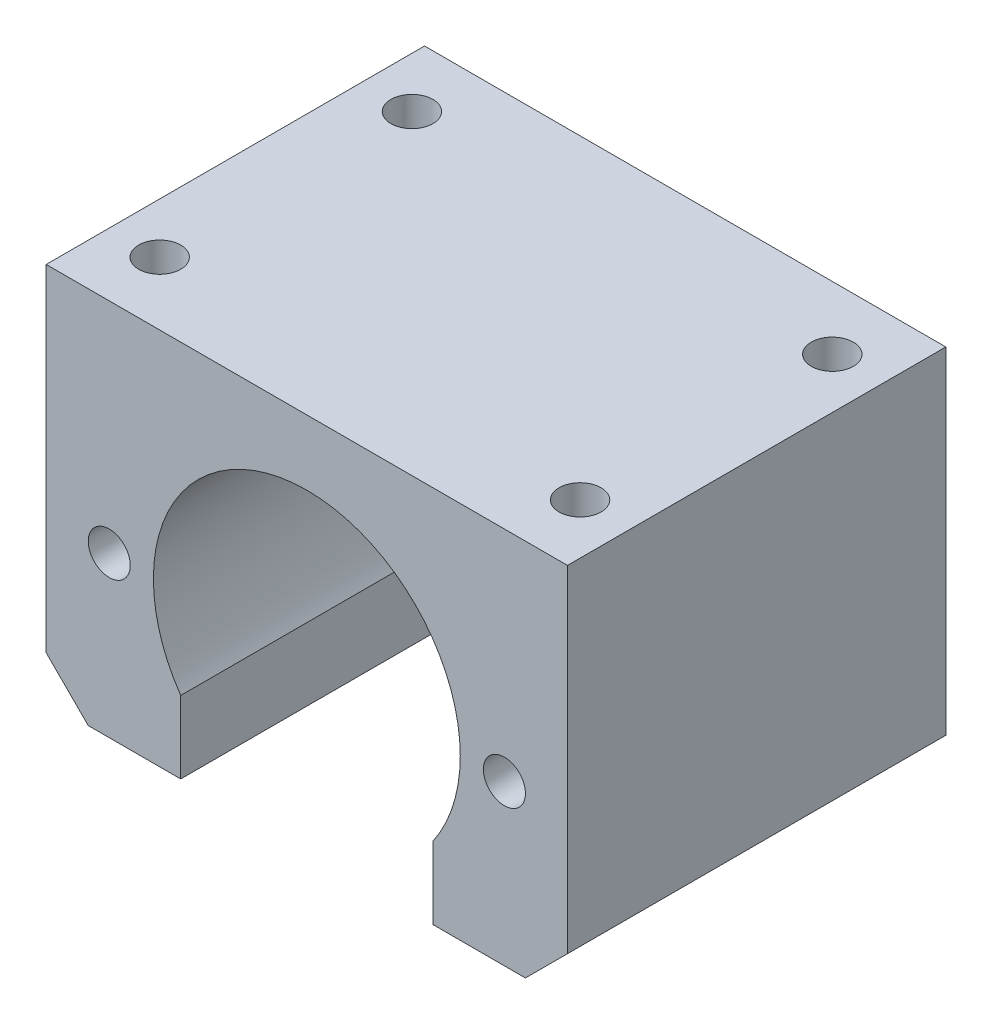
SolidWorks part; units mm, degrees
material "A6061"
ref_plane "前基準面" through (0, 0, 0) normal (0, 0, 1) x (1, 0, 0)
ref_plane "上基準面" through (0, 0, 0) normal (0, 1, 0) x (1, 0, 0)
ref_plane "右基準面" through (0, 0, 0) normal (1, 0, 0) x (0, 0, -1)
sketch "草图1" plane through (0, 0, 0) normal (0, 1, 0) x (1, 0, 0)
  line L1 (-31, -22.5) -> (31, -22.5)
  line L2 (-31, -22.5) -> (-31, 22.5)
  line L3 (-31, 22.5) -> (31, 22.5)
  line L4 (31, -22.5) -> (31, 22.5)
  line L5 (-31, -22.5) -> (31, 22.5) construction
  line L6 (-31, 22.5) -> (31, -22.5) construction
  point P0 (0, 0)
  dimension "D1" = 62
  dimension "D2" = 45
extrude "凸台-拉伸1" add sketch "草图1" along normal mid plane 45
sketch "草图2" plane through (0, 0, -22.5) normal (0, 0, -1) x (-1, 0, 0)
  line L0 (-31, 22.5) -> (31, 22.5) construction
  line L1 (-31, -22.5) -> (31, -22.5) construction
  line L3 (-15, -13.8953) -> (-15, -22.5)
  line L4 (-15, -22.5) -> (15, -22.5)
  line L5 (15, -13.8953) -> (15, -22.5)
  arc A0 (15, -13.8953) -> (-15, -13.8953) centre (0, -3.5) ccw
  dimension "D1" = 36.5
  dimension "D2" = 26
  dimension "D3" = 30
extrude "切除-拉伸1" cut sketch "草图2" against normal up to surface (45 mm away) up to face at (0, 0, 22.5)
chamfer "倒角1" distance 5 angle 45 2 edges at (31, -22.5, 0) (-31, -22.5, 0)
hole_wizard "M6 螺纹孔1" positions "草图3" profile "草图4" tap size "M6" standard "GB"
sketch "草图3" plane through (0, 22.5, 0) normal (0, 1, 0) x (1, 0, 0)
  line L0 (0, 27.8605) -> (0, 0) construction
  line L1 (0, 0) -> (-41.3894, 0) construction
  point P0 (-25, 15)
  point P9 (-25, -15)
  point P10 (25, -15)
  point P11 (25, 15)
  dimension "D1" = 30
  dimension "D2" = 50
sketch "草图4" plane through (-25, 22.5, -15) normal (1, 0, 0) x (0, 0, 1)
  line L0 (0, 0) -> (0, 16.5022)
  line L1 (0, 16.5022) -> (2.5, 15)
  line L2 (2.5, 15) -> (2.5, 0)
  line L5 (2.5, 0) -> (0, 0)
  line L10 (0, 16.5022) -> (-2.5, 15) construction
  line L11 (0, -6.35) -> (0, 107.95) construction
  dimension "螺纹孔钻头直径" = 5
  dimension "螺纹孔钻头深度" = 15
  dimension "导头角度" = 118
cosmetic thread "孔螺蚊线1" parameters "D1"=12, "D2"=6
cosmetic thread "孔螺蚊线2" parameters "D1"=12, "D2"=6
cosmetic thread "孔螺蚊线3" parameters "D1"=12, "D2"=6
cosmetic thread "孔螺蚊线4" parameters "D1"=12, "D2"=6
hole_wizard "M6 螺纹孔2" positions "草图5" profile "草图6" tap size "M6" standard "GB"
sketch "草图5" plane through (0, 0, -22.5) normal (0, 0, -1) x (-1, 0, 0)
  line L0 (0, 20.303) -> (0, -3.5) construction
  point P0 (-23.5, -3.5)
  point P6 (23.5, -3.5)
  dimension "D1" = 47
sketch "草图6" plane through (23.5, -3.5, -22.5) normal (1, 0, 0) x (0, 1, 0)
  line L0 (0, 0) -> (0, 16.5022)
  line L1 (0, 16.5022) -> (2.5, 15)
  line L2 (2.5, 15) -> (2.5, 0)
  line L5 (2.5, 0) -> (0, 0)
  line L10 (0, 16.5022) -> (-2.5, 15) construction
  line L11 (0, -6.35) -> (0, 107.95) construction
  dimension "螺纹孔钻头直径" = 5
  dimension "螺纹孔钻头深度" = 15
  dimension "导头角度" = 118
cosmetic thread "孔螺蚊线5" parameters "D1"=12, "D2"=6
cosmetic thread "孔螺蚊线6" parameters "D1"=12, "D2"=6
mirror "镜向1" about plane through (0, 0, 0) normal (0, 0, 1) of "M6 螺纹孔2"
